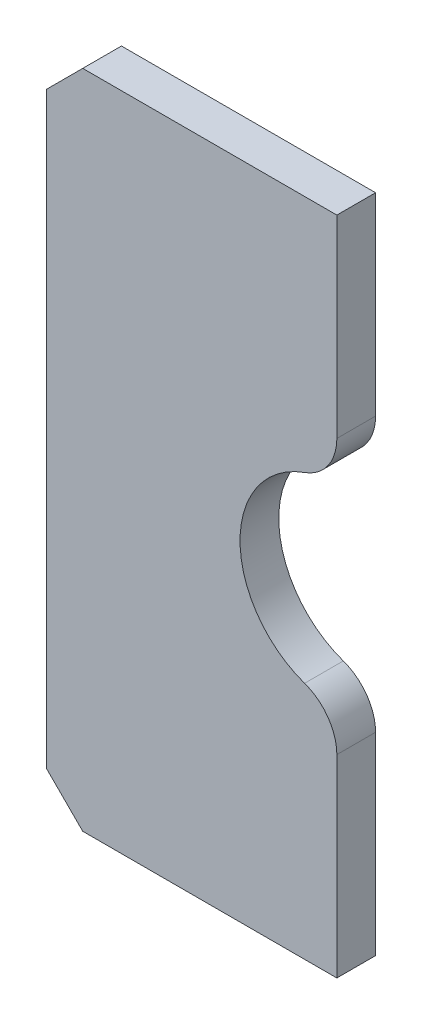
SolidWorks part; units mm, degrees
ref_plane "Front Plane" through (0, 0, 0) normal (0, 0, 1) x (1, 0, 0)
ref_plane "Top Plane" through (0, 0, 0) normal (0, 1, 0) x (1, 0, 0)
ref_plane "Right Plane" through (0, 0, 0) normal (1, 0, 0) x (0, 0, -1)
sketch "Sketch1" plane through (0, 0, 0) normal (0, 0, 1) x (1, 0, 0)
  line L0 (0, 258) -> (15, 273)
  line L1 (15, 0) -> (120, 0)
  line L2 (0, 15) -> (0, 258)
  line L3 (15, 273) -> (120, 273)
  line L4 (120, 0) -> (120, 79.9315)
  line L5 (15, 0) -> (0, 15)
  line L6 (120, 193.0685) -> (120, 273)
  arc A0 (106.6667, 174.2124) -> (106.6667, 98.7876) centre (120, 136.5) ccw
  arc A1 (120, 79.9315) -> (106.6667, 98.7876) centre (100, 79.9315) ccw
  arc A2 (120, 193.0685) -> (106.6667, 174.2124) centre (100, 193.0685) cw
  point P0 (0, 0)
  point P2 (0, 273)
  point P16 (120, 176.5)
  dimension "D3" = 80
  dimension "D10" = 20
  dimension "D1" = 120
  dimension "D2" = 273
  dimension "D4" = 15
  dimension "D5" = 45
  dimension "D6" = 15
  dimension "D7" = 45
  dimension "D8" = 136.5
  dimension "D9" = 120
extrude "Boss-Extrude1" add sketch "Sketch1" along normal blind 16
